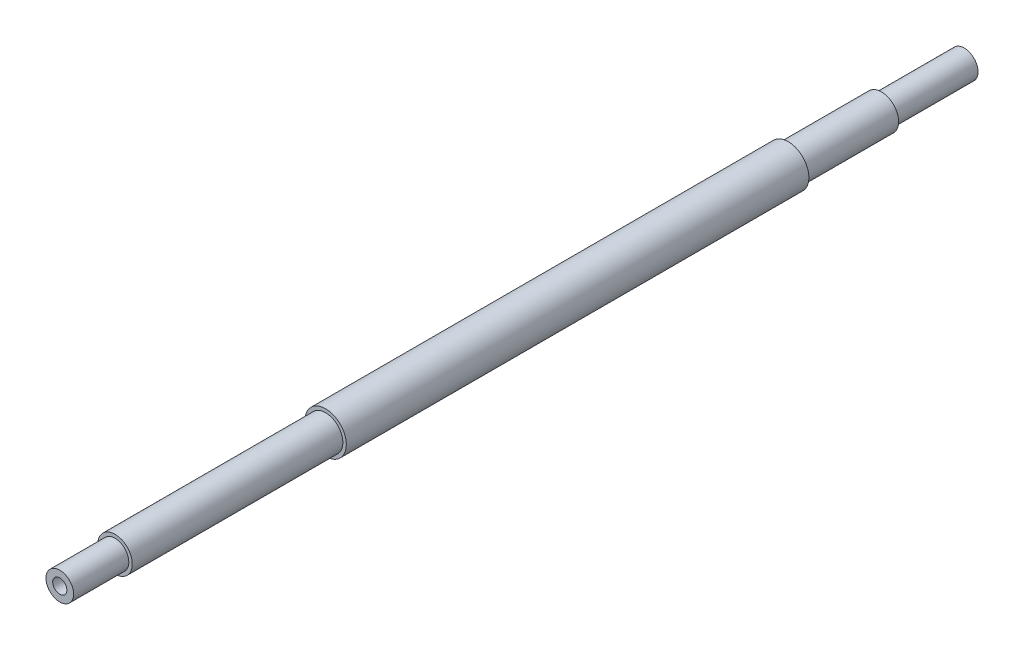
from build123d import *

# Parameters (mm, degrees)
SKETCH1_R               = 2.5
BOSS_EXTRUDE1_DEPTH     = 13.5
SKETCH2_R               = 3
BOSS_EXTRUDE2_DEPTH     = 67
SKETCH3_R               = 2.5
BOSS_EXTRUDE3_DEPTH     = 30.5
SKETCH4_R               = 2
BOSS_EXTRUDE4_DEPTH     = 8
BOSS_EXTRUDE5_START     = 12
SKETCH5_R               = 2
BOSS_EXTRUDE5_DEPTH     = 12
M2_5_TAPPED_HOLE1_D     = 2.05
M2_5_TAPPED_HOLE1_DEPTH = 6.35
M2_5_TAPPED_HOLE1_TIP   = 0.615882135


with BuildPart() as part:
    # Sketch1 → Boss-Extrude1 (new body)
    with BuildSketch(Plane.XY):
        Circle(SKETCH1_R)
    extrude(amount=BOSS_EXTRUDE1_DEPTH)

    # Sketch2 → Boss-Extrude2 (add)
    with BuildSketch(Plane.XY.offset(13.5)):
        Circle(SKETCH2_R)
    extrude(amount=BOSS_EXTRUDE2_DEPTH)

    # Sketch3 → Boss-Extrude3 (add)
    with BuildSketch(Plane.XY.offset(80.5)):
        Circle(SKETCH3_R)
    extrude(amount=BOSS_EXTRUDE3_DEPTH)

    # Sketch4 → Boss-Extrude4 (add)
    with BuildSketch(Plane.XY.offset(111)):
        Circle(SKETCH4_R)
    extrude(amount=BOSS_EXTRUDE4_DEPTH)

    # Sketch5 → Boss-Extrude5 (add)
    with BuildSketch(Plane(origin=(0, 0, 0), x_dir=(-1, 0, 0), z_dir=(0, 0, -1)).offset(BOSS_EXTRUDE5_START)):
        with Locations(Location((0, 0, 0), (0, 0, 180))):
            Circle(SKETCH5_R)
    extrude(amount=-BOSS_EXTRUDE5_DEPTH)

    # M2.5 Tapped Hole1
    with Locations(Plane.XY.offset(119)):
        with Locations((0, 0)):
            Hole(M2_5_TAPPED_HOLE1_D / 2, depth=M2_5_TAPPED_HOLE1_DEPTH)
            with Locations((0, 0, -(M2_5_TAPPED_HOLE1_DEPTH + M2_5_TAPPED_HOLE1_TIP / 2))):  # 118° drill point
                Cone(0, M2_5_TAPPED_HOLE1_D / 2, M2_5_TAPPED_HOLE1_TIP, mode=Mode.SUBTRACT)


solid = part.part
